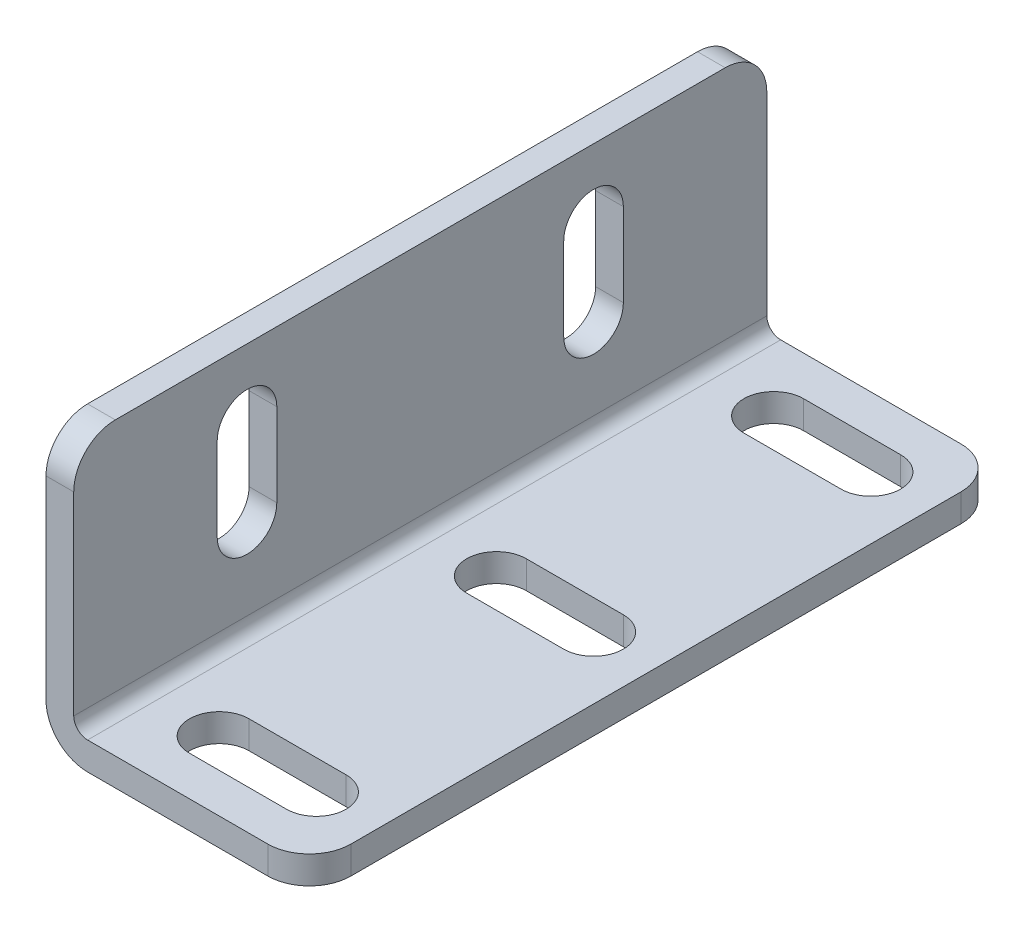
from build123d import *

# Parameters (mm, degrees)
EXTRUDE_1_DEPTH     = 25
CUT_EXTRUDE_1_DEPTH = 10
CUT_EXTRUDE_2_DEPTH = 10
FILLET_1_R          = 3
FILLET_2_R          = 1
FILLET_3_R          = 3


with BuildPart() as part:
    # 草图9 → 拉伸-薄壁1 (new, symmetric)
    with BuildSketch(Plane.XY):
        Polygon((17, 0), (0, 0), (0, 18), (-2, 18), (-2, -2), (17, -2), align=None)
    extrude(amount=EXTRUDE_1_DEPTH, both=True)

    # 草图10 → 切除-拉伸1 (cut)
    with BuildSketch(Plane(origin=(0, 0, 0), x_dir=(1, 0, 0), z_dir=(0, 1, 0))):
        with BuildLine():
            Line((5.5, 22.15), (12.5, 22.15))
            ThreePointArc((12.5, 22.15), (14.65, 20), (12.5, 17.85))
            Line((12.5, 17.85), (5.5, 17.85))
            ThreePointArc((5.5, 17.85), (3.35, 20), (5.5, 22.15))
        make_face()
        with BuildLine():
            Line((5.5, -22.15), (12.5, -22.15))
            ThreePointArc((12.5, -22.15), (14.65, -20), (12.5, -17.85))
            Line((12.5, -17.85), (5.5, -17.85))
            ThreePointArc((5.5, -17.85), (3.35, -20), (5.5, -22.15))
        make_face()
        with BuildLine():
            Line((5.5, 2.15), (12.5, 2.15))
            ThreePointArc((12.5, 2.15), (14.65, 0), (12.5, -2.15))
            Line((12.5, -2.15), (5.5, -2.15))
            ThreePointArc((5.5, -2.15), (3.35, 0), (5.5, 2.15))
        make_face()
    extrude(amount=-CUT_EXTRUDE_1_DEPTH, mode=Mode.SUBTRACT)

    # 草图11 → 切除-拉伸2 (cut)
    with BuildSketch(Plane(origin=(0, 0, 0), x_dir=(0, 0, -1), z_dir=(1, 0, 0))):
        with BuildLine():
            Line((-10.35, 13), (-10.35, 7))
            ThreePointArc((-10.35, 7), (-12.5, 4.85), (-14.65, 7))
            Line((-14.65, 7), (-14.65, 13))
            ThreePointArc((-14.65, 13), (-12.5, 15.15), (-10.35, 13))
        make_face()
        with BuildLine():
            Line((10.35, 13), (10.35, 7))
            ThreePointArc((10.35, 7), (12.5, 4.85), (14.65, 7))
            Line((14.65, 7), (14.65, 13))
            ThreePointArc((14.65, 13), (12.5, 15.15), (10.35, 13))
        make_face()
    extrude(amount=-CUT_EXTRUDE_2_DEPTH, mode=Mode.SUBTRACT)

    # 圆角1
    fillet_1_edges = [part.edges().sort_by_distance(p)[0] for p in [
        (-1, 18, 25),
        (-1, 18, -25),
        (17, -1, -25),
        (17, -1, 25),
    ]]
    fillet(fillet_1_edges, radius=FILLET_1_R)

    # 圆角2
    fillet_2_edges = [part.edges().sort_by_distance(p)[0] for p in [
        (0, 0, 0),
    ]]
    fillet(fillet_2_edges, radius=FILLET_2_R)

    # 圆角3
    fillet_3_edges = [part.edges().sort_by_distance(p)[0] for p in [
        (-2, -2, 0),
    ]]
    fillet(fillet_3_edges, radius=FILLET_3_R)


solid = part.part
